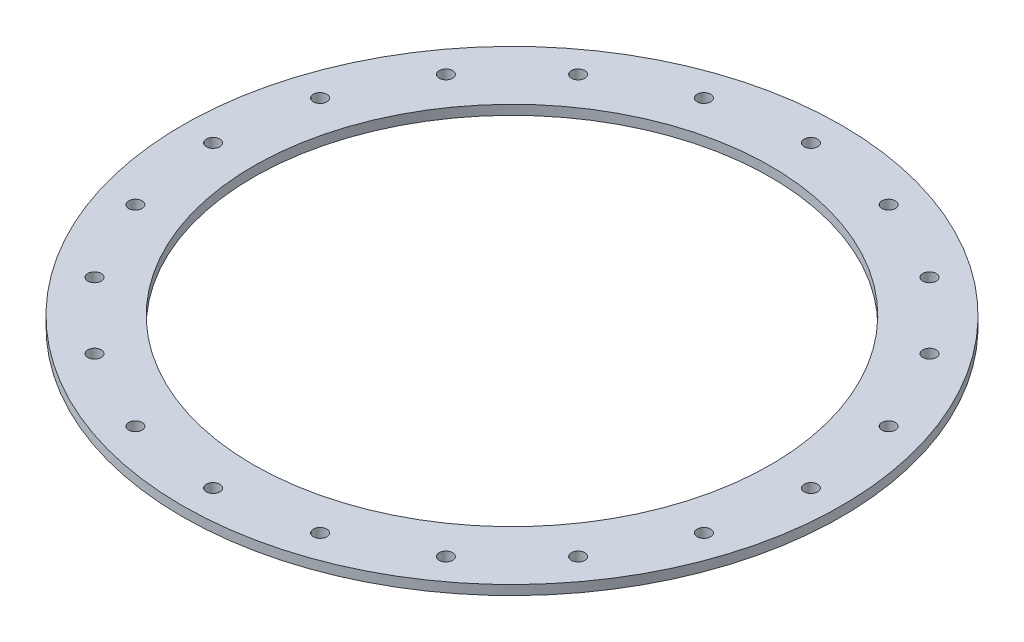
from build123d import *

# Parameters (mm, degrees)
SKETCH_1_R                = 860
SKETCH_1_R_2              = 675
EXTRUDE_1_DEPTH           = 25
HOLE_WIZARD_25_5_25_5_1_D = 35


with BuildPart() as part:
    # 草图1 → 凸台-拉伸1 (new body)
    with BuildSketch(Plane(origin=(0, 0, 0), x_dir=(1, 0, 0), z_dir=(0, 1, 0))):
        with Locations(Location((0, 0, 0), (0, 0, 270))):
            Circle(SKETCH_1_R)
        with Locations(Location((0, 0, 0), (0, 0, 270))):
            Circle(SKETCH_1_R_2, mode=Mode.SUBTRACT)
    extrude(amount=EXTRUDE_1_DEPTH)

    # Ø25.5 (25.5) 直径孔1 (through all)
    with Locations(Plane(origin=(0, 25, 0), x_dir=(1, 0, 0), z_dir=(0, 1, 0))):
        with Locations((0, 780), (241.033255612, 741.82408271), (458.472496788, 631.033255612), (631.033255612, 458.472496788), (741.82408271, 241.033255612), (780, 0), (741.82408271, -241.033255612), (631.033255612, -458.472496788), (458.472496788, -631.033255612), (241.033255612, -741.82408271), (0, -780), (-241.033255612, -741.82408271), (-458.472496788, -631.033255612), (-631.033255612, -458.472496788), (-741.82408271, -241.033255612), (-780, 0), (-741.82408271, 241.033255612), (-631.033255612, 458.472496788), (-458.472496788, 631.033255612), (-241.033255612, 741.82408271)):
            Hole(HOLE_WIZARD_25_5_25_5_1_D / 2)


solid = part.part
